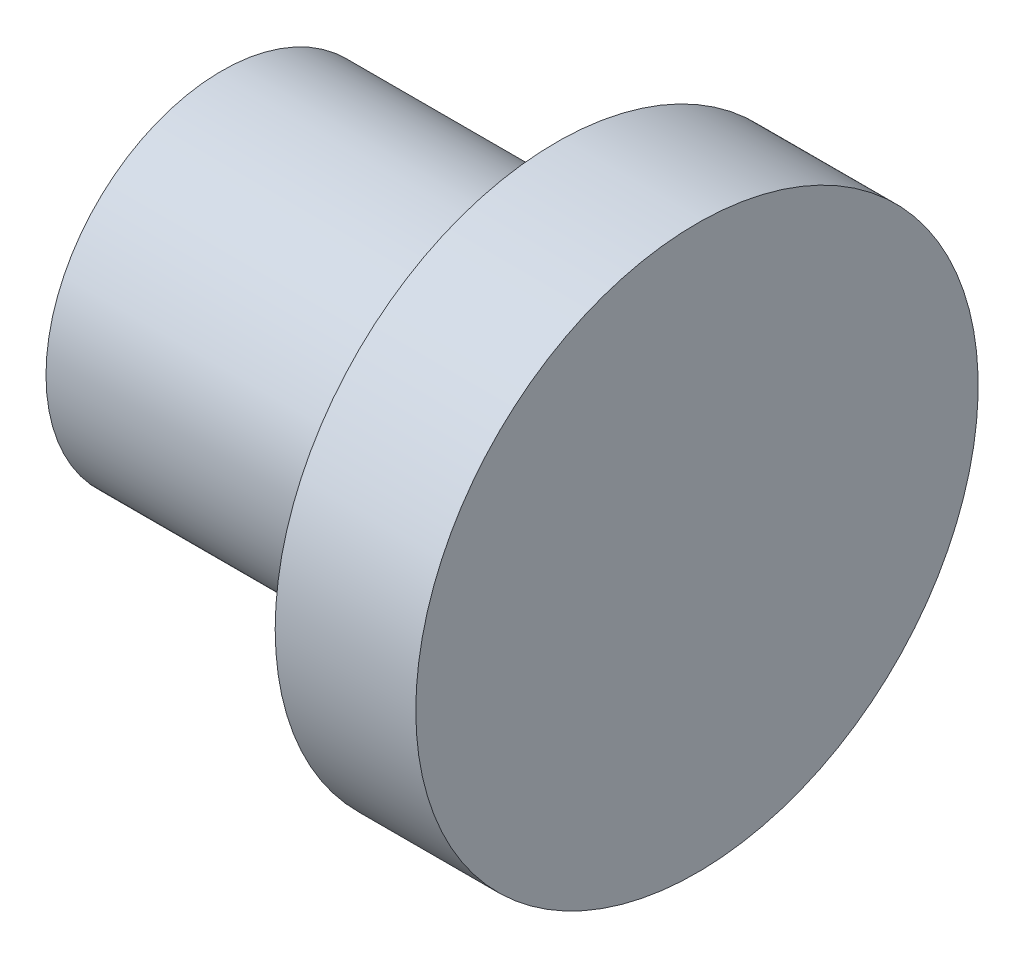
from build123d import *


with BuildPart() as part:
    # Sketch1 → Revolve1 (revolve)
    with BuildSketch(Plane.XY, mode=Mode.PRIVATE) as revolve1_sk:
        Polygon((-585.02727965, -122.37788349), (-573.12727965, -122.37788349), (-573.12727965, -126.12788349), (-568.12727965, -126.12788349), (-568.12727965, -116.12788349), (-585.02727965, -116.12788349), align=None)
    revolve(revolve1_sk.sketch.rotate(Axis((-585.02727965, -116.12788349, 0), (1, 0, 0)), 270), axis=Axis((-585.02727965, -116.12788349, 0), (1, 0, 0)))


solid = part.part
